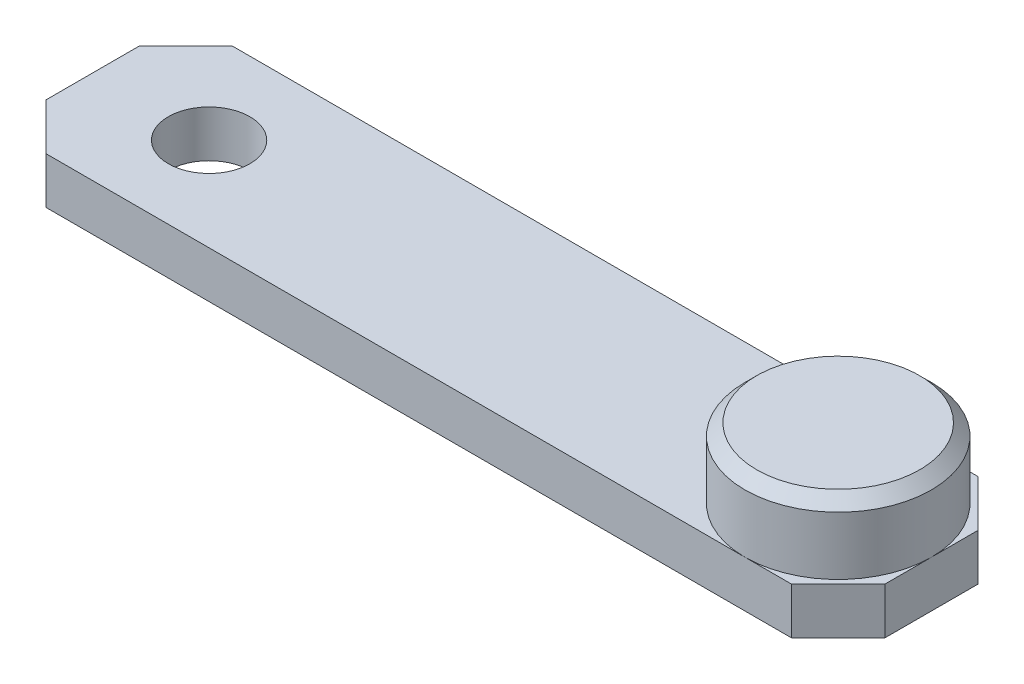
SolidWorks part; units mm, degrees
ref_plane "Front Plane" through (0, 0, 0) normal (0, 0, 1) x (1, 0, 0)
ref_plane "Top Plane" through (0, 0, 0) normal (0, 1, 0) x (1, 0, 0)
ref_plane "Right Plane" through (0, 0, 0) normal (1, 0, 0) x (0, 0, -1)
sketch "Sketch1" plane through (0, 0, 0) normal (0, 1, 0) x (1, 0, 0)
  line L1 (0, 8) -> (36, 8)
  line L2 (0, 8) -> (0, 0)
  line L3 (0, 0) -> (36, 0)
  line L4 (36, 8) -> (36, 0)
  dimension "D1" = 36
  dimension "D2" = 8
extrude "Boss-Extrude1" add sketch "Sketch1" along normal blind 2
sketch "Sketch2" plane through (0, 2, 0) normal (0, 1, 0) x (1, 0, 0)
  line L0 (36, 8) -> (0, 8) construction
  line L1 (0, 8) -> (0, 0) construction
  circle A0 centre (5, 4) radius 1.75
  dimension "D3" = 3.5
  dimension "D1" = 4
  dimension "D2" = 5
extrude "Cut-Extrude1" cut sketch "Sketch2" against normal through all
sketch "Sketch3" plane through (0, 2, 0) normal (0, 1, 0) x (1, 0, 0)
  line L0 (36, 8) -> (0, 8) construction
  line L1 (36, 0) -> (36, 8) construction
  circle A0 centre (32, 4) radius 4
  dimension "D2" = 4
  dimension "D3" = 8
  dimension "D1" = 4
extrude "Boss-Extrude2" add sketch "Sketch3" along normal blind 3
chamfer "Chamfer1" distance 0.5 angle 45 1 edges at (32, 5, 0)
chamfer "Chamfer2" distance 2 angle 45 4 edges at (36, 1, -8) (36, 1, 0) (0, 1, 0) (0, 1, -8)
